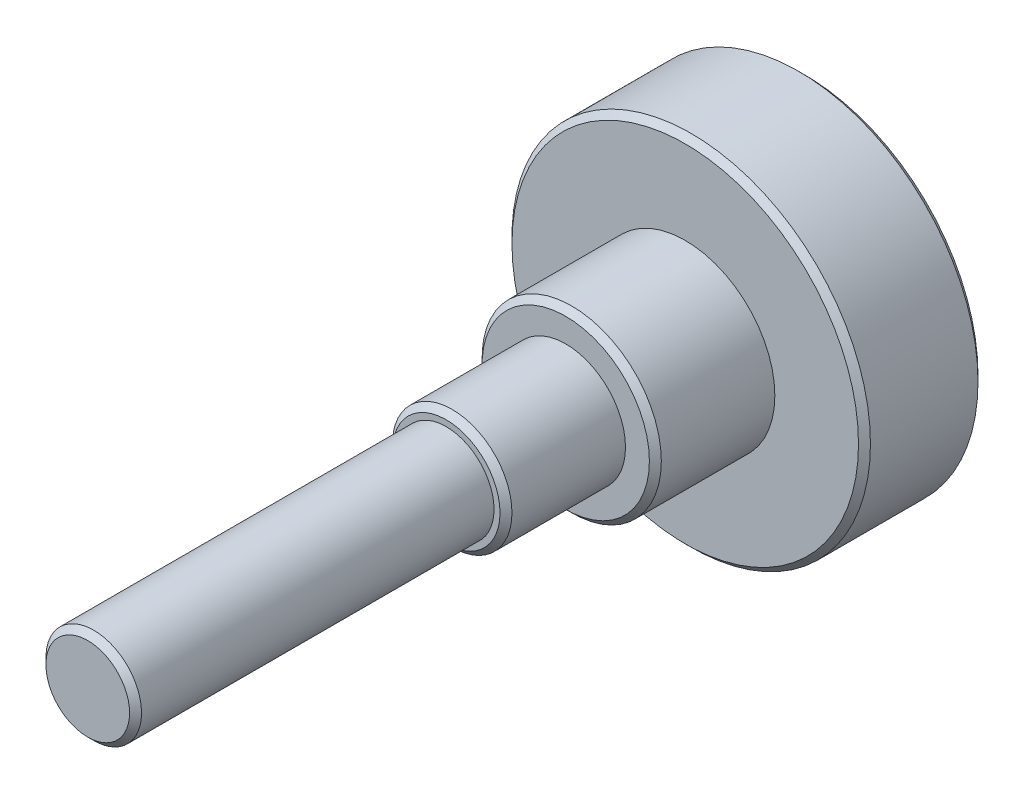
from build123d import *

# Parameters (mm, degrees)
SKETCH1_R           = 15
BOSS_EXTRUDE1_DEPTH = 10
SKETCH2_R           = 7.5
BOSS_EXTRUDE2_DEPTH = 10
SKETCH3_R           = 4
BOSS_EXTRUDE3_DEPTH = 40
SKETCH4_R           = 5
BOSS_EXTRUDE4_DEPTH = 10
CHAMFER1_SIZE       = 0.5


with BuildPart() as part:
    # Sketch1 → Boss-Extrude1 (new body)
    with BuildSketch(Plane.XY):
        Circle(SKETCH1_R)
    extrude(amount=BOSS_EXTRUDE1_DEPTH)

    # Sketch2 → Boss-Extrude2 (add)
    with BuildSketch(Plane.XY.offset(10)):
        Circle(SKETCH2_R)
    extrude(amount=BOSS_EXTRUDE2_DEPTH)

    # Sketch3 → Boss-Extrude3 (add)
    with BuildSketch(Plane.XY.offset(20)):
        Circle(SKETCH3_R)
    extrude(amount=BOSS_EXTRUDE3_DEPTH)

    # Sketch4 → Boss-Extrude4 (add)
    with BuildSketch(Plane.XY.offset(20)):
        Circle(SKETCH4_R)
    extrude(amount=BOSS_EXTRUDE4_DEPTH)

    # Chamfer1
    chamfer1_edges = [part.edges().sort_by_distance(p)[0] for p in [
        (-4, 0, 60),
        (-5, 0, 30),
        (-15, 0, 0),
        (-15, 0, 10),
        (-7.5, 0, 20),
    ]]
    chamfer(chamfer1_edges, length=CHAMFER1_SIZE)


solid = part.part
